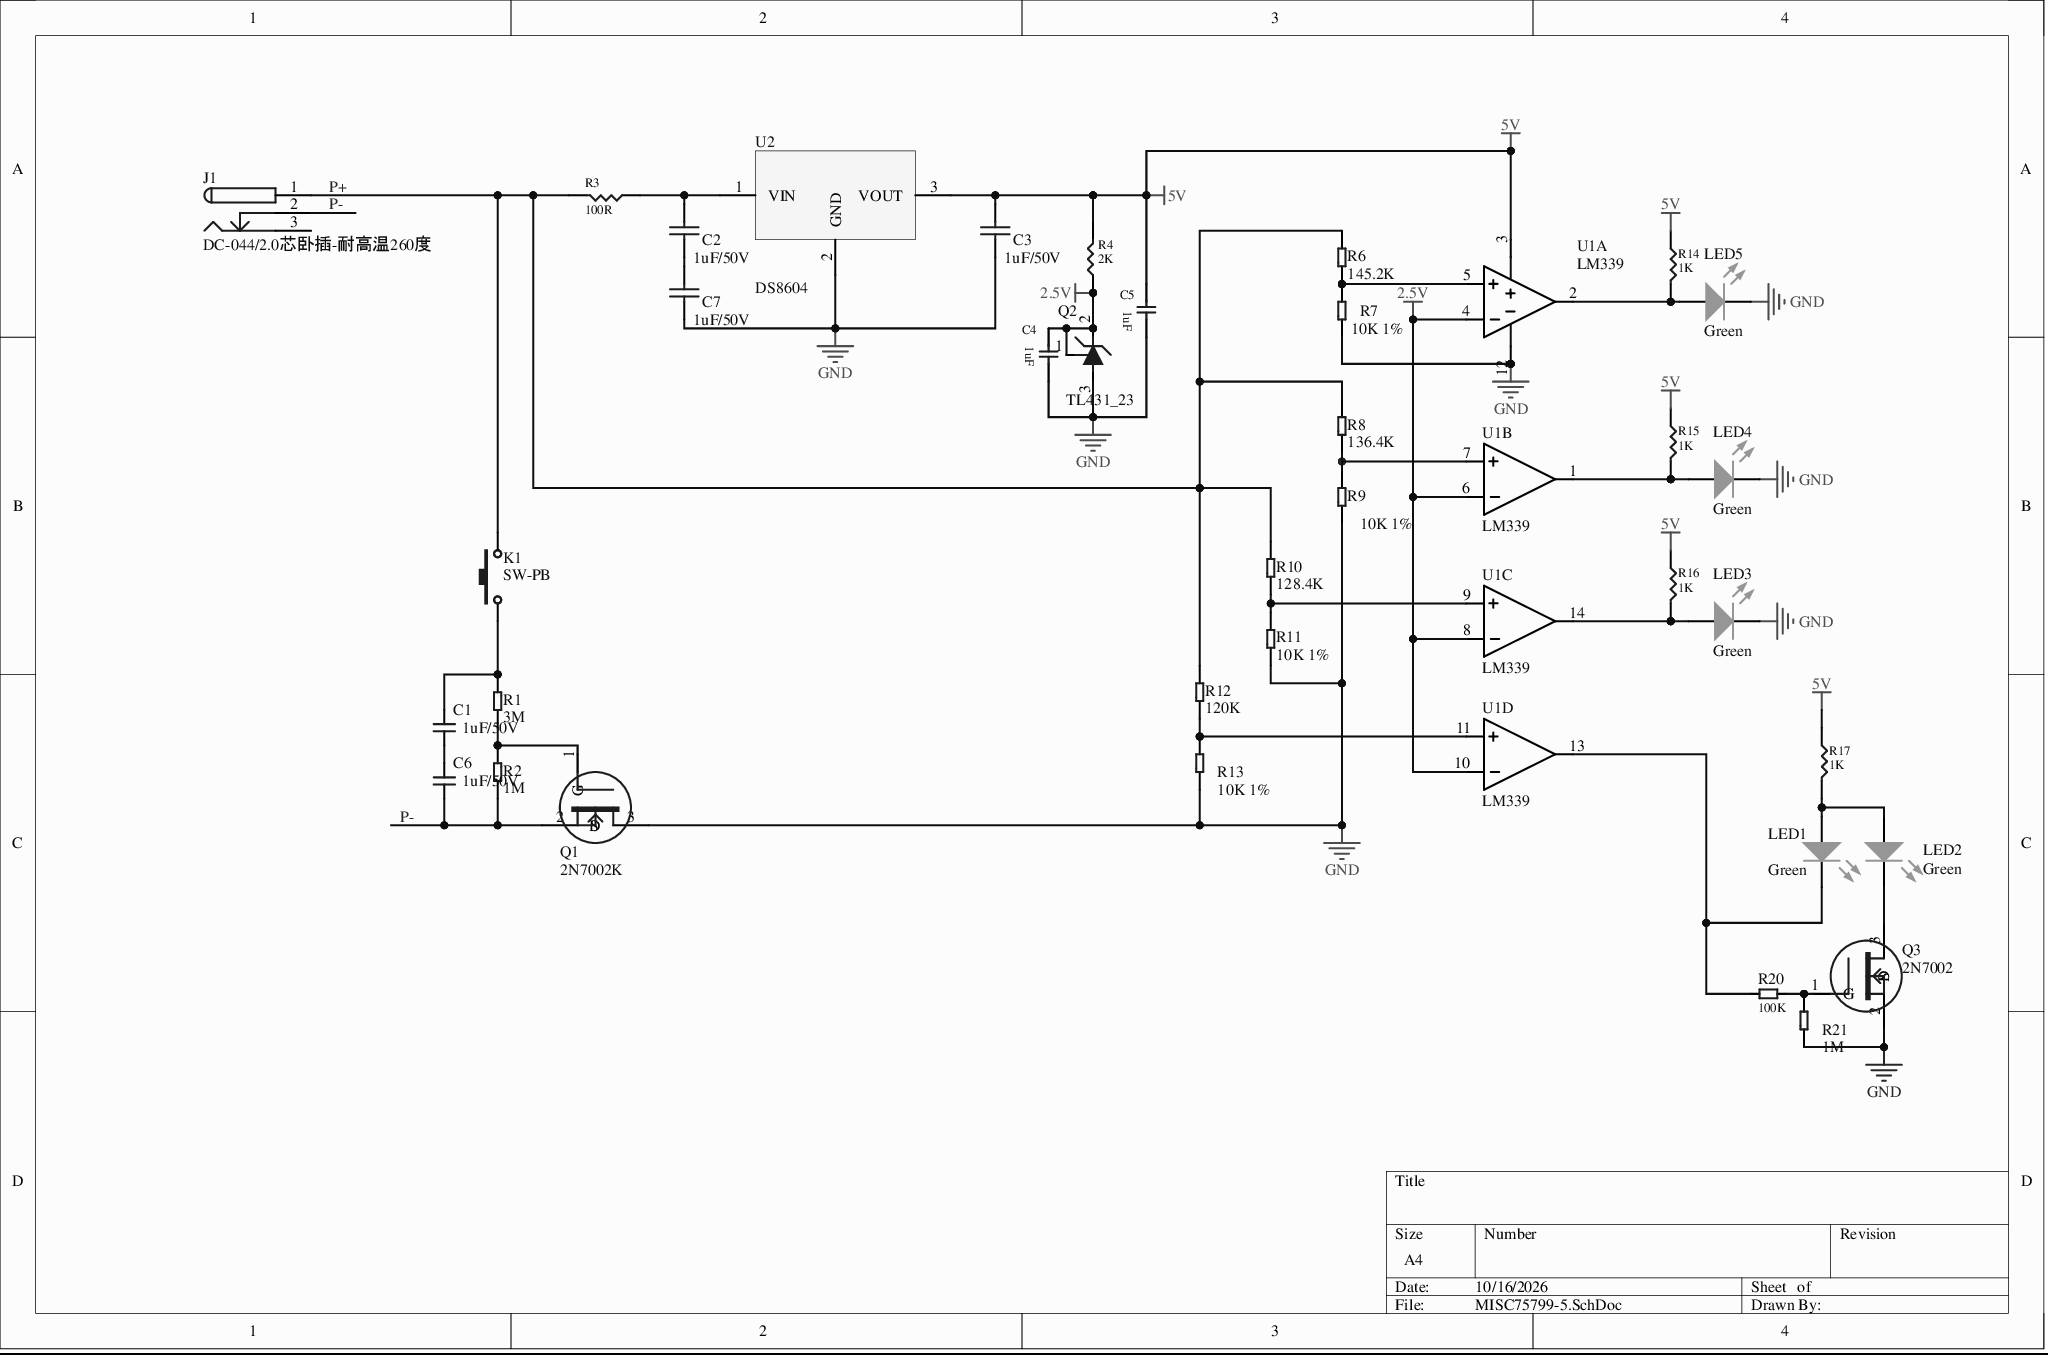
[diagram p0: MISC75799-5.SchDoc]
# Altium project MISC75799-3.PrjPcb
1 sheet, 37 parts. Net scope: global (net labels, ports and power ports of the same name join across sheets).
Board file: MISC75799.PcbDoc

## Sheet MISC75799-5.SchDoc
size A4; SheetNumber: 1; SheetTotal: 1

### Parts
C1  1uF/50V  [C0603A]
C2  1uF/50V  [C0603A]
C3  1uF/50V  [C0603A]
C4  1uF  [C0603A]
C5  1uF  [C0603A]
C6  1uF/50V  [C0603A]
C7  1uF/50V  [C0603A]
J1  DC-044/2.0芯卧插-耐高温260度  [DC-044]
K1  SW-PB  [SW-SMD_4P-L12.0-W12.0-P5.00-LS15.2]
LED1  Green  [LED0603A]
LED2  Green  [LED0603A]
LED3  Green  [LED0603A]
LED4  Green  [LED0603A]
LED5  Green  [LED0603A]
Q1  2N7002K  [SOT23-3]
Q2  TL431_23  [SOT23-3]
Q3  2N7002  [SOT23-3]
R1  3M  [R0603A]
R2  1M  [R0603A]
R3  100R  [R0805A]
R4  2K  [R0805A]
R6  145.2K  [R0603A]
R7  10K 1%  [R0603A]
R8  136.4K  [R0603A]
R9  10K 1%  [R0603A]
R10  128.4K  [R0603A]
R11  10K 1%  [R0603A]
R12  120K  [R0603A]
R13  10K 1%  [R0603A]
R14  1K  [R0603A]
R15  1K  [R0603A]
R16  1K  [R0603A]
R17  1K  [R0603A]
R20  100K  [R0603A]
R21  1M  [R0603A]
U1  LM339  [SOP14L]  (parts A,B,C,D of 4)
U2  DS8604  [SOT-89-3]

### Nets
2.5V: C4.2 Q2.1 Q2.2 R4.1 U1.4(IN1-) U1.6(IN2-) U1.8(IN3-) U1.10(IN4-)
5V: C3.2 C5.2 R4.2 R14.1 R15.1 R16.1 R17.1 U1.3(VCC) U2.3(VOUT)
GND: C3.1 C4.1 C5.1 C7.1 LED3.1(A) LED4.1(A) LED5.1(A) Q1.3(D) Q2.3 Q3.2(S) R7.1 R9.1 R11.1 R13.1 R21.1 U1.12(GND) U2.2(GND)
P+: J1.1 K1.2 R3.2 R6.2 R8.2 R10.2 R12.2
P-: C6.2 J1.2 Q1.2(S) R2.2
NetC1_1: C1.1 K1.1 R1.1
NetC1_2: C1.2 C6.1
NetC2_1: C2.1 C7.2
NetC2_2: C2.2 R3.1 U2.1(VIN)
NetLED1_1: LED1.1(A) R20.2 U1.13(OUT4)
NetLED1_2: LED1.2(K) LED2.2(K) R17.2
NetLED2_1: LED2.1(A) Q3.3(D)
NetLED3_2: LED3.2(K) R16.2 U1.14(OUT3)
NetLED4_2: LED4.2(K) R15.2 U1.1(OUT2)
NetLED5_2: LED5.2(K) R14.2 U1.2(OUT1)
NetQ1_1: Q1.1(G) R1.2 R2.1
NetQ3_1: Q3.1(G) R20.1 R21.2
NetR6_1: R6.1 R7.2 U1.5(IN1+)
NetR8_1: R8.1 R9.2 U1.7(IN2+)
NetR10_1: R10.1 R11.2 U1.9(IN3+)
NetR12_1: R12.1 R13.2 U1.11(IN4+)

Not connected (* = marked no-connect by the designer): J1 3

### Library data of the parts
C1 C6 = C0603: 0603 SMD capacitor
C2 C3 C7 = Cap: Capacitor; Published: 8-Jun-2000; LatestRevisionDate: 17-Jul-2002; LatestRevisionNote: Re-released for DXP Platform.; PackageReference: RAD-0.3; PackageDescription: Radial Cap, Thru-Hole; 2 Leads; 0.3 in Pin Spacing; Publisher: Altium Limited
C4 C5 = 0.1u
J1 = DC-044/2.0芯卧插-耐高温260度: DC-044 power connector - Yueqing Jinghong
K1 = SW-PB_1: 6*6 tactile switch; Published: 24-Mar-1999; LatestRevisionDate: 17-Jul-2002; LatestRevisionNote: Re-released for DXP Platform.; PackageReference: SPST-2; PackageDescription: Switch; 2 Leads; Publisher: Altium Limited
LED1-LED5 = LED_Green: SMD LED lamp
Q1 Q3 = NMOS
Q2 = TL431_23: IC SOT-23
R1 R2 R6-R13 R21 = R
R3 R4 R14-R17 = RES
R20 = R-S
U2 = LDO DS8604: LDO